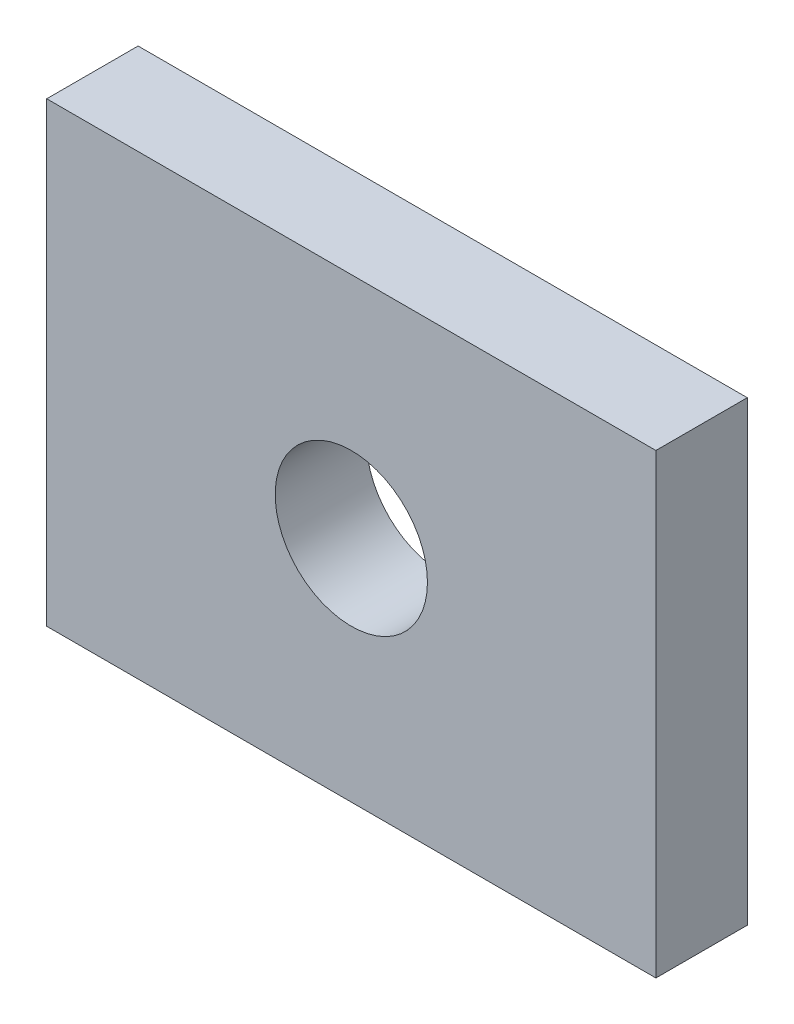
from build123d import *

# Parameters (mm, degrees)
SKETCH1_W           = 40
SKETCH1_H           = 30
BOSS_EXTRUDE1_DEPTH = 6
SKETCH2_R           = 5
CUT_EXTRUDE1_DEPTH  = 6


with BuildPart() as part:
    # Sketch1 → Boss-Extrude1 (new body)
    with BuildSketch(Plane.XY):
        with Locations((-26.669019685, -3.132226563)):
            Rectangle(SKETCH1_W, SKETCH1_H)
    extrude(amount=BOSS_EXTRUDE1_DEPTH)

    # Sketch2 → Cut-Extrude1 (cut)
    with BuildSketch(Plane.XY.offset(6)):
        with Locations((-26.669019685, -3.132226563)):
            Circle(SKETCH2_R)
    extrude(amount=-CUT_EXTRUDE1_DEPTH, mode=Mode.SUBTRACT)


solid = part.part
